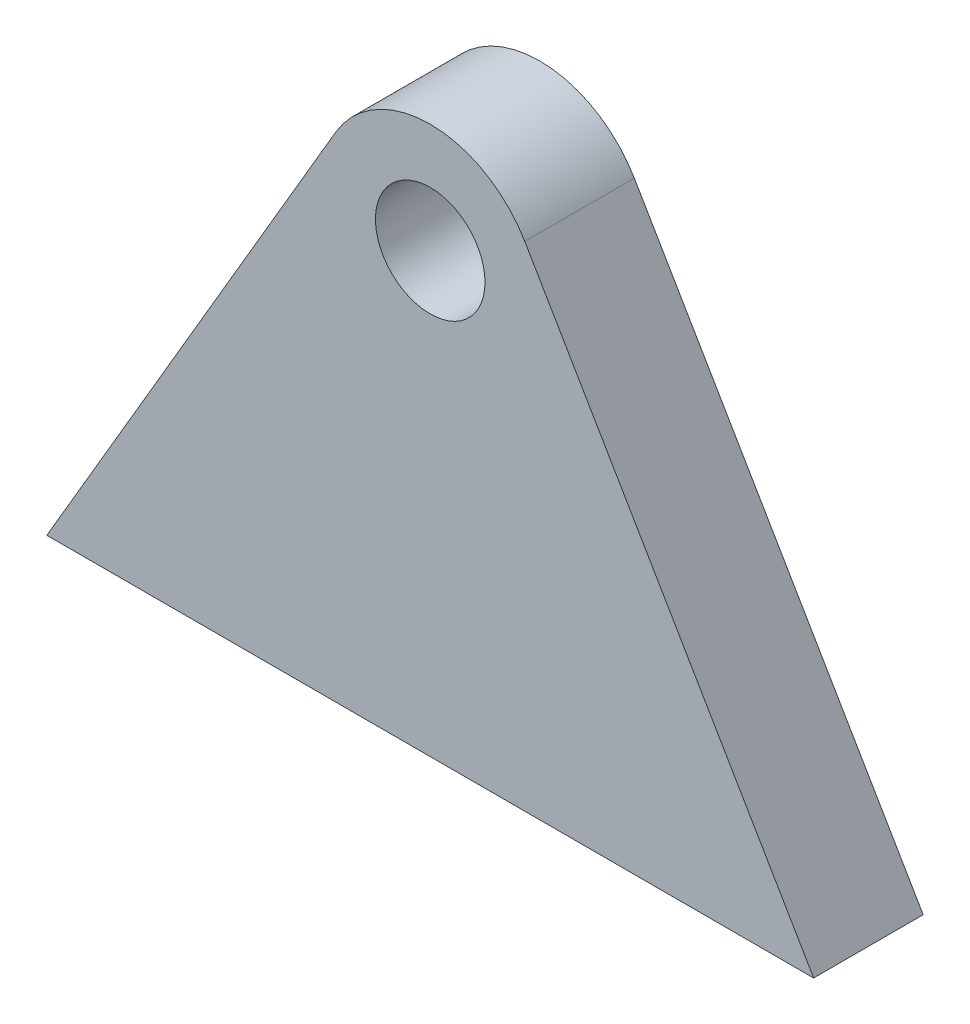
SolidWorks part; units mm, degrees
material "普通碳钢"
ref_plane "Front Plane" through (0, 0, 0) normal (0, 0, 1) x (1, 0, 0)
ref_plane "Top Plane" through (0, 0, 0) normal (0, 1, 0) x (1, 0, 0)
ref_plane "Right Plane" through (0, 0, 0) normal (1, 0, 0) x (0, 0, -1)
sketch "Sketch1" plane through (0, 0, 0) normal (0, 0, 1) x (1, 0, 0)
  line L0 (-35, -40) -> (35, -40)
  line L3 (-35, -40) -> (-8.6303, 5.0515)
  line L4 (35, -40) -> (8.6303, 5.0515)
  circle A0 centre (0, 0) radius 5
  arc A1 (8.6303, 5.0515) -> (-8.6303, 5.0515) centre (0, 0) ccw
  dimension "D4" = 10
  dimension "D5" = 10
  dimension "D2" = 40
  dimension "D1" = 70
extrude "Boss-Extrude1" add sketch "Sketch1" along normal blind 10
